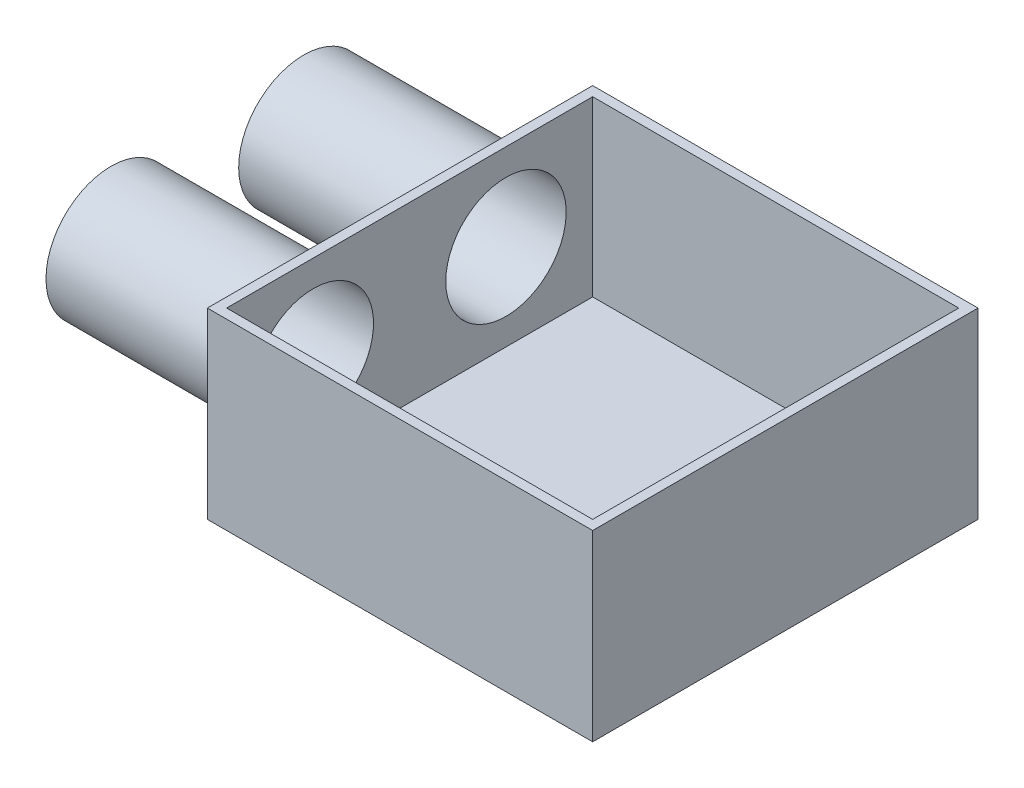
SolidWorks part; units mm, degrees
ref_plane "Front Plane" through (0, 0, 0) normal (0, 0, 1) x (1, 0, 0)
ref_plane "Top Plane" through (0, 0, 0) normal (0, 1, 0) x (1, 0, 0)
ref_plane "Right Plane" through (0, 0, 0) normal (1, 0, 0) x (0, 0, -1)
sketch "Sketch1" plane through (0, 0, 0) normal (0, 1, 0) x (1, 0, 0)
  line L1 (-40, 40) -> (40, 40)
  line L2 (-40, 40) -> (-40, -40)
  line L3 (-40, -40) -> (40, -40)
  line L4 (40, 40) -> (40, -40)
  line L5 (-40, 40) -> (40, -40) construction
  line L6 (-40, -40) -> (40, 40) construction
  point P0 (0, 0)
  dimension "D1" = 80
  dimension "D2" = 80
extrude "Boss-Extrude1" add sketch "Sketch1" along normal blind 38
sketch "Sketch2" plane through (0, 38, 0) normal (0, 1, 0) x (1, 0, 0)
  line L0 (40, 40) -> (-40, 40) construction
  line L1 (-38, -38) -> (38, -38)
  line L2 (-38, -38) -> (-38, 38)
  line L3 (-38, 38) -> (38, 38)
  line L4 (38, -38) -> (38, 38)
  line L5 (-38, -38) -> (38, 38) construction
  line L6 (-38, 38) -> (38, -38) construction
  line L7 (-40, 40) -> (-40, -40) construction
  point P0 (0, 0)
  dimension "D1" = 2
  dimension "D2" = 2
extrude "Cut-Extrude1" cut sketch "Sketch2" against normal blind 36
sketch "Sketch3" plane through (-40, 0, 0) normal (-1, 0, 0) x (0, 0, 1)
  line L0 (-40, 38) -> (40, 38) construction
  line L1 (0, 0) -> (0, 48.4099) construction
  circle A0 centre (-20, 20) radius 12.5
  circle A1 centre (20, 20) radius 12.5
  dimension "D1" = 25
  dimension "D2" = 18
  dimension "D3" = 40
extrude "Cut-Extrude2" cut sketch "Sketch3" against normal blind 10
sketch "Sketch4" plane through (-40, 0, 0) normal (-1, 0, 0) x (0, 0, 1)
  circle A0 centre (-20, 20) radius 12.5 construction
  circle A1 centre (-20, 20) radius 12.5
  circle A2 centre (20, 20) radius 12.5 construction
  circle A3 centre (20, 20) radius 12.5
  circle A4 centre (-20, 20) radius 13.5
  circle A5 centre (20, 20) radius 13.5
  dimension "D1" = 1
extrude "Boss-Extrude3" add sketch "Sketch4" along normal blind 40
